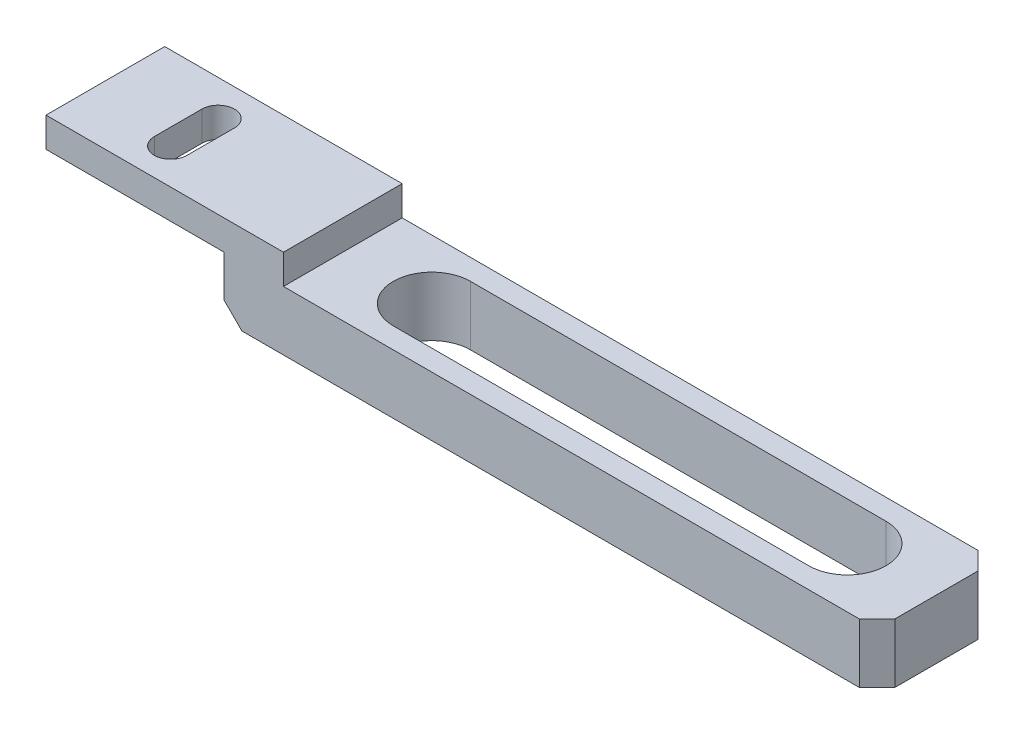
from build123d import *

# Parameters (mm, degrees)
EXTRUDE_1_DEPTH     = 10
CUT_EXTRUDE_1_DEPTH = 142.155942135
CUT_EXTRUDE_2_DEPTH = 142.155942135
CHAMFER_1_SIZE      = 3
CHAMFER_2_SIZE      = 3
SKETCH_5_W          = 100
SKETCH_5_H          = 5
CUT_EXTRUDE_3_DEPTH = 143.214626533


with BuildPart() as part:
    # 草图2 → 凸台-拉伸1 (new, symmetric)
    with BuildSketch(Plane.XY):
        Polygon((0, 0), (140, 0), (140, -15), (30, -15), (30, -5), (0, -5), align=None)
    extrude(amount=EXTRUDE_1_DEPTH, both=True)

    # 草图3 → 切除-拉伸1 (cut, through all)
    with BuildSketch(Plane(origin=(0, 0, 0), x_dir=(1, 0, 0), z_dir=(0, 1, 0))):
        with BuildLine():
            Line((55, 6.5), (125, 6.5))
            ThreePointArc((125, 6.5), (131.5, 0), (125, -6.5))
            Line((125, -6.5), (55, -6.5))
            ThreePointArc((55, -6.5), (48.5, 0), (55, 6.5))
        make_face()
    extrude(amount=-CUT_EXTRUDE_1_DEPTH, mode=Mode.SUBTRACT)

    # 草图4 → 切除-拉伸2 (cut, through all)
    with BuildSketch(Plane(origin=(0, 0, 0), x_dir=(1, 0, 0), z_dir=(0, 1, 0))):
        with BuildLine():
            Line((17.75, 4), (17.75, -4))
            ThreePointArc((17.75, -4), (15, -6.75), (12.25, -4))
            Line((12.25, -4), (12.25, 4))
            ThreePointArc((12.25, 4), (15, 6.75), (17.75, 4))
        make_face()
    extrude(amount=-CUT_EXTRUDE_2_DEPTH, mode=Mode.SUBTRACT)

    # 倒角1
    chamfer_1_edges = [part.edges().sort_by_distance(p)[0] for p in [
        (140, -7.5, 10),
        (140, -7.5, -10),
    ]]
    chamfer(chamfer_1_edges, length=CHAMFER_1_SIZE)

    # 倒角2
    chamfer_2_edges = [part.edges().sort_by_distance(p)[0] for p in [
        (30, -15, 0),
    ]]
    chamfer(chamfer_2_edges, length=CHAMFER_2_SIZE)

    # 草图5 → 切除-拉伸3 (cut, through all)
    with BuildSketch(Plane.XY.offset(10)):
        with Locations((90, -2.5)):
            Rectangle(SKETCH_5_W, SKETCH_5_H)
    extrude(amount=-CUT_EXTRUDE_3_DEPTH, mode=Mode.SUBTRACT)


solid = part.part
